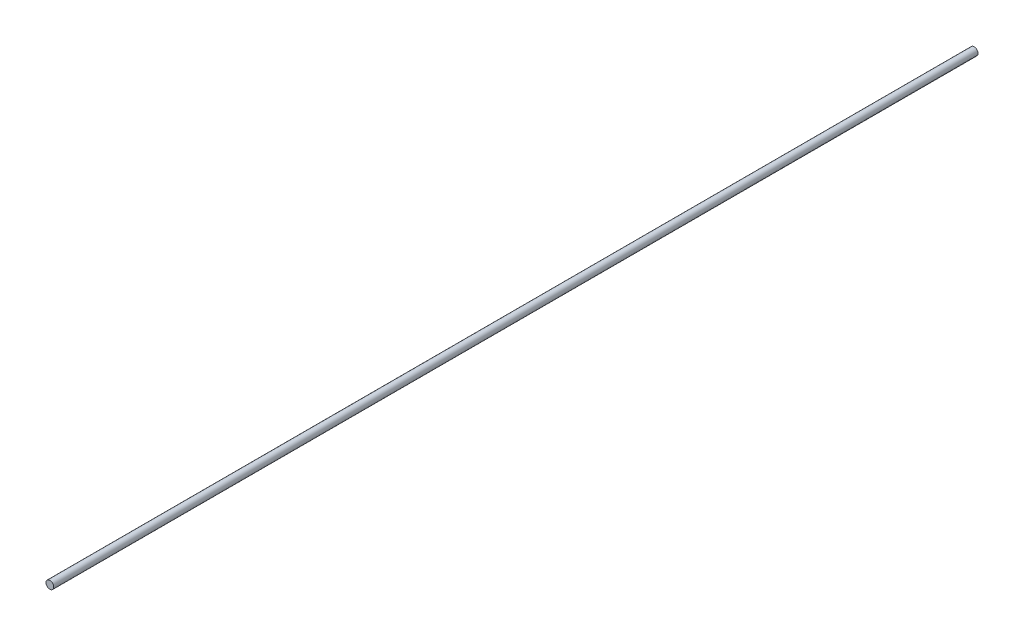
SolidWorks part; units mm, degrees
material "SWM-B"
ref_plane "Front Plane" through (0, 0, 0) normal (0, 0, 1) x (1, 0, 0)
ref_plane "Top Plane" through (0, 0, 0) normal (0, 1, 0) x (1, 0, 0)
ref_plane "Right Plane" through (0, 0, 0) normal (1, 0, 0) x (0, 0, -1)
sketch "Sketch1" plane through (0, 0, 0) normal (0, 0, 1) x (1, 0, 0)
  circle A0 centre (0, 0) radius 2
  dimension "D1" = 4
extrude "Boss-Extrude1" add sketch "Sketch1" along normal blind 479.4
